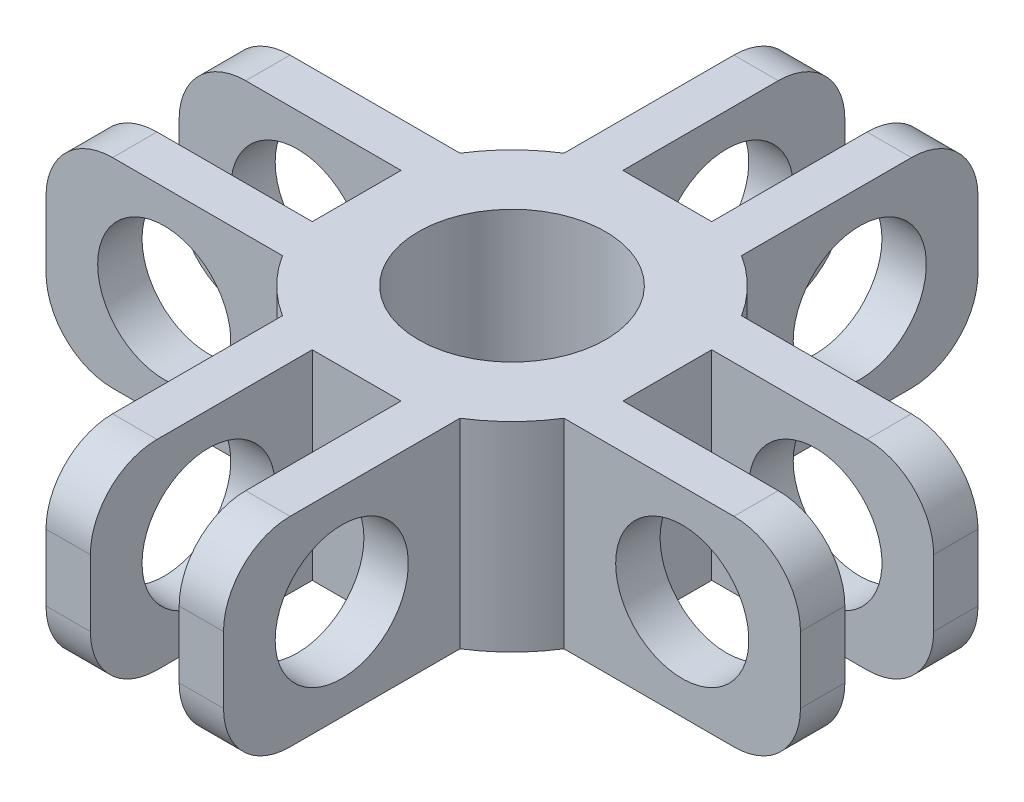
SolidWorks part; units mm, degrees
ref_plane "Front Plane" through (0, 0, 0) normal (0, 0, 1) x (1, 0, 0)
ref_plane "Top Plane" through (0, 0, 0) normal (0, 1, 0) x (1, 0, 0)
ref_plane "Right Plane" through (0, 0, 0) normal (1, 0, 0) x (0, 0, -1)
sketch "Sketch1" plane through (0, 0, 0) normal (0, 1, 0) x (1, 0, 0)
  line L0 (0, 25.1724) -> (0, -25.4316) construction
  line L1 (-5.08, 21.59) -> (5.08, 21.59)
  line L2 (-21.59, -5.08) -> (-21.59, 5.08)
  line L3 (-5.08, -21.59) -> (5.08, -21.59)
  line L4 (21.59, 5.08) -> (21.59, -5.08)
  line L5 (-5.08, 5.08) -> (5.08, -5.08) construction
  line L6 (-5.08, -5.08) -> (5.08, 5.08) construction
  line L7 (-46.9715, 0) -> (29.8892, 0) construction
  line L9 (-21.59, 5.08) -> (-5.08, 5.08)
  line L10 (-5.08, 21.59) -> (-5.08, 5.08)
  line L15 (21.59, 5.08) -> (5.08, 5.08)
  line L16 (5.08, 21.59) -> (5.08, 5.08)
  line L21 (21.59, -5.08) -> (5.08, -5.08)
  line L22 (5.08, -21.59) -> (5.08, -5.08)
  line L27 (-21.59, -5.08) -> (-5.08, -5.08)
  line L28 (-5.08, -21.59) -> (-5.08, -5.08)
  point P0 (0, 0)
  dimension "D1" = 5.08
  dimension "D2" = 5.08
  dimension "D3" = 5.08
  dimension "D4" = 5.08
  dimension "D5" = 21.59
  dimension "D6" = 21.59
  dimension "D7" = 21.59
  dimension "D8" = 5.08
  dimension "D9" = 5.08
  dimension "D10" = 21.59
extrude "Boss-Extrude1" add sketch "Sketch1" along normal blind 11.43
sketch "Sketch2" plane through (0, 11.43, 0) normal (0, 1, 0) x (1, 0, 0)
  circle A0 centre (0, 0) radius 9.525
  dimension "D1" = 19.05
extrude "Boss-Extrude2" add sketch "Sketch2" against normal up to surface (11.43 mm away) up to face at (0, 0, 0)
sketch "Sketch8" plane through (-5.08, 0, 0) normal (-1, 0, 0) x (0, 0, 1)
  line L0 (14.8236, 11.43) -> (14.8236, 5.715) construction
  line L1 (8.0572, 11.43) -> (21.59, 11.43) construction
  line L2 (14.8236, 5.715) -> (21.59, 5.715) construction
  line L3 (21.59, 11.43) -> (21.59, 0) construction
  line L4 (-14.8236, 5.715) -> (-14.8236, 11.43) construction
  line L5 (-21.59, 11.43) -> (-8.0572, 11.43) construction
  line L6 (-14.8236, 11.43) -> (-14.8236, 5.715) construction
  line L7 (-14.8236, 5.715) -> (-21.59, 5.715) construction
  line L8 (-21.59, 11.43) -> (-21.59, 0) construction
  circle A0 centre (14.8236, 5.715) radius 3.81
  circle A1 centre (-14.8236, 5.715) radius 3.81
  dimension "D1" = 7.62
  dimension "D2" = 7.62
extrude "Cut-Extrude6" cut sketch "Sketch8" against normal through all
sketch "Sketch9" plane through (0, 0, -5.08) normal (0, 0, -1) x (-1, 0, 0)
  line L0 (14.8236, 5.715) -> (21.59, 5.715) construction
  line L1 (21.59, 11.43) -> (21.59, 0) construction
  line L2 (14.8236, 5.715) -> (14.8236, 11.43) construction
  line L3 (8.0572, 11.43) -> (21.59, 11.43) construction
  line L4 (-14.8236, 5.715) -> (-14.8236, 11.43) construction
  line L5 (-21.59, 11.43) -> (-8.0572, 11.43) construction
  line L6 (-14.8236, 5.715) -> (-21.59, 5.715) construction
  line L7 (-21.59, 11.43) -> (-21.59, 0) construction
  circle A0 centre (14.8236, 5.715) radius 3.81
  circle A1 centre (-14.8236, 5.715) radius 3.81
  dimension "D1" = 7.62
  dimension "D2" = 7.62
extrude "Cut-Extrude7" cut sketch "Sketch9" against normal through all
hole_wizard "1/2-13 Tapped Hole1" positions "Sketch11" profile "Sketch10" tap size "1/2-13" standard "ANSI Inch" end condition through all
sketch "Sketch11" plane through (0, 11.43, 0) normal (0, 1, 0) x (1, 0, 0)
  point P0 (0, 0)
sketch "Sketch10" plane through (0, 11.43, 0) normal (1, 0, 0) x (0, 0, 1)
  line L0 (0, 0) -> (0, 11.43)
  line L1 (0, 11.43) -> (5.3581, 11.43)
  line L2 (5.3581, 11.43) -> (5.3581, 0)
  line L5 (5.3581, 0) -> (0, 0)
  line L11 (0, -6.35) -> (0, 107.95) construction
  dimension "Thru Tap Drill Dia." = 10.7163
  dimension "Thru Tap Drill Depth" = 11.43
cosmetic thread "Hole Thread5" parameters "D2"=12.7
sketch "Sketch12" plane through (0, 11.43, 0) normal (0, 1, 0) x (1, 0, 0)
  line L0 (-21.59, 5.08) -> (-21.59, -5.08) construction
  line L1 (-8.89, 2.54) -> (-34.29, 2.54)
  line L2 (-8.89, 2.54) -> (-8.89, -2.54)
  line L3 (-8.89, -2.54) -> (-34.29, -2.54)
  line L4 (-34.29, 2.54) -> (-34.29, -2.54)
  line L5 (-8.89, 2.54) -> (-34.29, -2.54) construction
  line L6 (-8.89, -2.54) -> (-34.29, 2.54) construction
  line L7 (-21.59, -5.08) -> (-8.0572, -5.08) construction
  point P0 (-21.59, 0)
  dimension "D1" = 12.7
  dimension "D2" = 2.54
extrude "Cut-Extrude8" cut sketch "Sketch12" against normal through all
pattern_circular "CirPattern1" count 4 every 90 about axis through (0, 0, 0) along (0, 1, 0) of "Cut-Extrude8"
fillet "Fillet1" radius 3.81 16 edges at (-3.81, 0, 21.59) (-3.81, 11.43, 21.59) (3.81, 11.43, 21.59) (3.81, 0, 21.59) (21.59, 11.43, 3.81) (21.59, 0, 3.81) (21.59, 11.43, -3.81) (21.59, 0, -3.81) (3.81, 0, -21.59) (3.81, 11.43, -21.59) (-3.81, 11.43, -21.59) (-3.81, 0, -21.59) (-21.59, 11.43, -3.81) (-21.59, 0, -3.81) (-21.59, 11.43, 3.81) (-21.59, 0, 3.81)
scale "Scale1" bodies to scale 116 scale about origin uniform scaling yes scale factor 2
